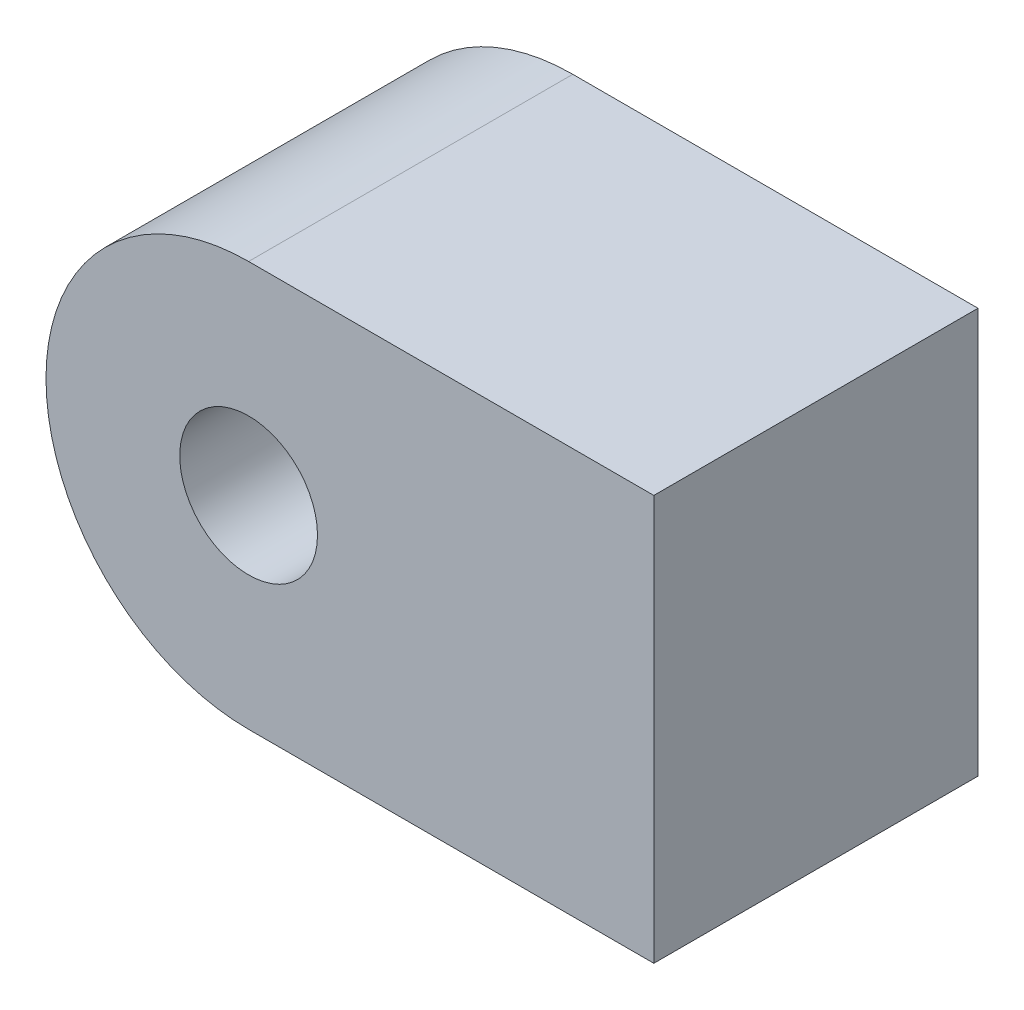
from build123d import *

# Parameters (mm, degrees)
SKETCH_1_R      = 5.1
EXTRUDE_1_DEPTH = 12


with BuildPart() as part:
    # 草图1 → 凸台-拉伸1 (new, symmetric)
    with BuildSketch(Plane.XY):
        with BuildLine():
            Line((0, 15), (30, 15))
            Line((30, 15), (30, -15))
            Line((30, -15), (0, -15))
            ThreePointArc((0, -15), (-15, 0), (0, 15))
        make_face()
        Circle(SKETCH_1_R, mode=Mode.SUBTRACT)
    extrude(amount=EXTRUDE_1_DEPTH, both=True)


solid = part.part
